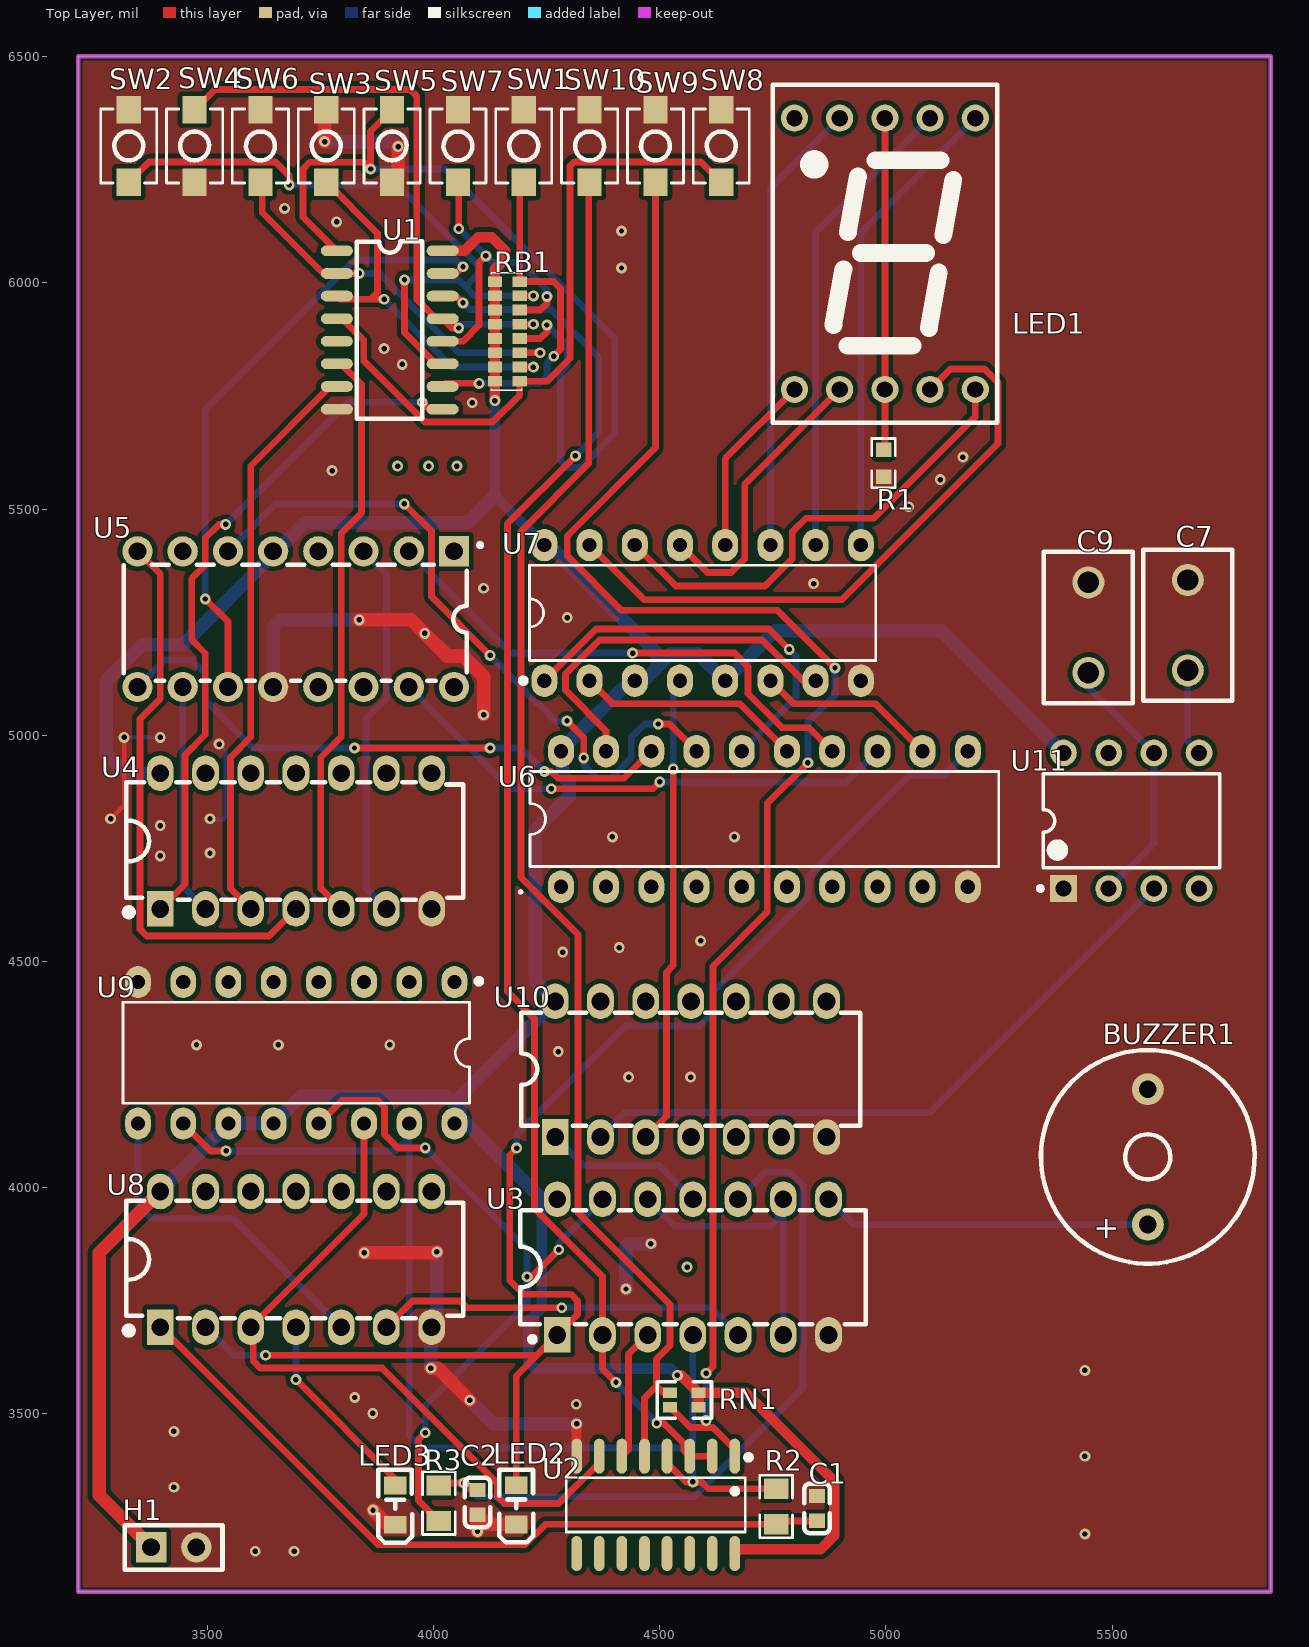
[diagram p0: Top Layer view]
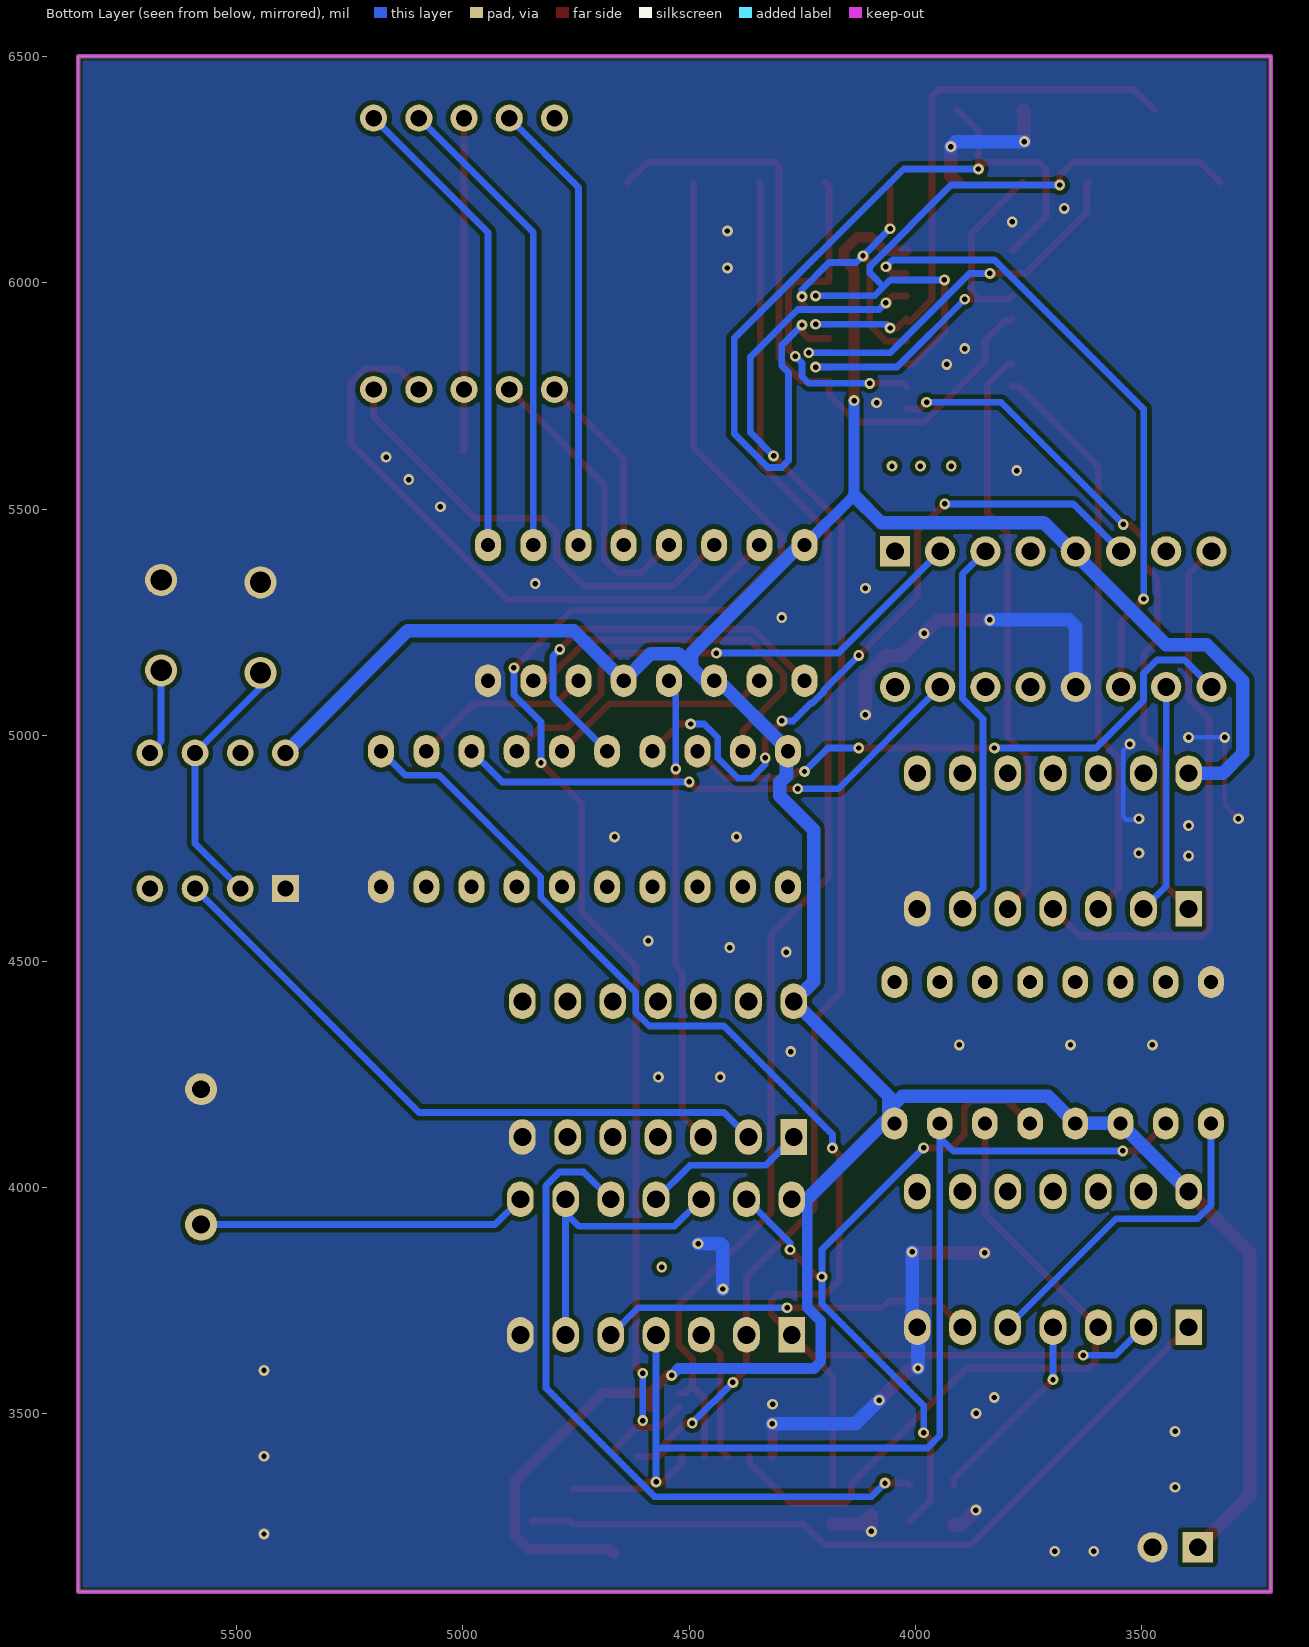
[diagram p1: Bottom Layer view, seen from below]
# Altium PCB MISC51700.pcbdoc
Units mil, origin at the board's own origin, x right, y up, seen from the top; angles counter-clockwise.
Board outline 2638.01 x 3396.77 mil, 2 copper layers (Top Layer, Bottom Layer), stack 62.206 mil thick; 35 components, 54 nets, 236 pads, 115 vias.

## Layer stack, top to bottom
Top Solder Mask Layer: solder mask 0.394, Dk 3.3
Top Layer: signal copper 1.379
Dielectric1: surface 59.449, FR4, Dk 4.5
Bottom Layer: signal copper 1.378
Bottom Solder Mask Layer: solder mask 0.394, Dk 3.3

## Board outline
3213.17,6501.82 3213.17,3105.05 5851.18,3105.05 5851.18,6501.82

## Design rules (kind name [scope] priority, off if disabled: settings)
BoardOutlineClearance copperThickness2oz_1 [All] p2 off: genericclearance=8 ignorepadtopadclearanceinfootprint=FALSE except(0: Arc-SplitContinuation Track-SplitContinuation SMDPad-SplitContinuation THPad-SplitContinuation Via-SplitContinuation Fill-SplitContinuation Region-SplitContinuation Poly-SplitContinuation Text-SplitContinuation Hole-SplitContinuation; 6: Arc-CutoutEdge Track-CutoutEdge SMDPad-CutoutEdge THPad-CutoutEdge Via-CutoutEdge Text-CutoutEdge; 6.9: Hole-OutlineEdge Hole-CutoutEdge; 10: Poly-OutlineEdge Poly-CutoutEdge; 11.8: Arc-OutlineEdge Track-OutlineEdge SMDPad-OutlineEdge THPad-OutlineEdge Via-OutlineEdge Fill-OutlineEdge Region-OutlineEdge Text-OutlineEdge Fill-CutoutEdge Region-CutoutEdge)
BoardOutlineClearance Plane_innerPlane_1 [All] p4 off: genericclearance=4 ignorepadtopadclearanceinfootprint=FALSE except(0: Arc-SplitContinuation Track-SplitContinuation SMDPad-SplitContinuation THPad-SplitContinuation Via-SplitContinuation Fill-SplitContinuation Region-SplitContinuation Poly-SplitContinuation Text-SplitContinuation Hole-SplitContinuation; 6: Arc-CutoutEdge Track-CutoutEdge SMDPad-CutoutEdge THPad-CutoutEdge Via-CutoutEdge Text-CutoutEdge; 6.9: Hole-OutlineEdge Hole-CutoutEdge; 10: Poly-OutlineEdge Poly-CutoutEdge; 11.8: Arc-OutlineEdge Track-OutlineEdge SMDPad-OutlineEdge THPad-OutlineEdge Via-OutlineEdge Fill-OutlineEdge Region-OutlineEdge Text-OutlineEdge Fill-CutoutEdge Region-CutoutEdge)
BoardOutlineClearance Copper_copperRegion_1 [All] p6 off: genericclearance=4 ignorepadtopadclearanceinfootprint=FALSE except(0: Arc-SplitContinuation Track-SplitContinuation SMDPad-SplitContinuation THPad-SplitContinuation Via-SplitContinuation Fill-SplitContinuation Region-SplitContinuation Poly-SplitContinuation Text-SplitContinuation Hole-SplitContinuation; 6: Arc-CutoutEdge Track-CutoutEdge SMDPad-CutoutEdge THPad-CutoutEdge Via-CutoutEdge Text-CutoutEdge; 6.9: Hole-OutlineEdge Hole-CutoutEdge; 10: Poly-OutlineEdge Poly-CutoutEdge; 11.8: Arc-OutlineEdge Track-OutlineEdge SMDPad-OutlineEdge THPad-OutlineEdge Via-OutlineEdge Fill-OutlineEdge Region-OutlineEdge Text-OutlineEdge Fill-CutoutEdge Region-CutoutEdge)
BoardOutlineClearance copperThickness1oz_1 [All] p8: genericclearance=4 ignorepadtopadclearanceinfootprint=FALSE except(0: Arc-SplitContinuation Track-SplitContinuation SMDPad-SplitContinuation THPad-SplitContinuation Via-SplitContinuation Fill-SplitContinuation Region-SplitContinuation Poly-SplitContinuation Text-SplitContinuation Hole-SplitContinuation; 6: Arc-CutoutEdge Track-CutoutEdge SMDPad-CutoutEdge THPad-CutoutEdge Via-CutoutEdge Text-CutoutEdge; 6.9: Hole-OutlineEdge Hole-CutoutEdge; 10: Poly-OutlineEdge Poly-CutoutEdge; 11.8: Arc-OutlineEdge Track-OutlineEdge SMDPad-OutlineEdge THPad-OutlineEdge Via-OutlineEdge Fill-OutlineEdge Region-OutlineEdge Text-OutlineEdge Fill-CutoutEdge Region-CutoutEdge)
Clearance copperThickness2oz [All] p1 off: gap=8 ignorepadtopadclearanceinfootprint=FALSE except(6: SMDPad-Track SMDPad-SMDPad THPad-Track SMDPad-THPad THPad-THPad Track-Via SMDPad-Via THPad-Via Via-Via Fill-SMDPad Region-SMDPad Fill-THPad Region-THPad Fill-Via Region-Via Fill-Fill Fill-Region Region-Region Arc-Track Arc-SMDPad Arc-THPad Arc-Via Fill-Arc Region-Arc Arc-Arc Text-Track SMDPad-Text Text-THPad Text-Via Fill-Text Region-Text Arc-Text Text-Text; 6.9: Hole-Track Hole-SMDPad Hole-THPad Hole-Via Fill-Hole Region-Hole Hole-Arc Hole-Text; 10: Poly-Track Poly-SMDPad Poly-THPad Poly-Via Poly-Fill Poly-Region Poly-Poly Poly-Arc Poly-Text Poly-Hole; 11.8: Fill-Track Region-Track)
Clearance Plane_innerPlane [All] p3 off: gap=4 ignorepadtopadclearanceinfootprint=FALSE except(6: SMDPad-Track SMDPad-SMDPad THPad-Track SMDPad-THPad THPad-THPad Track-Via SMDPad-Via THPad-Via Via-Via Fill-SMDPad Region-SMDPad Fill-THPad Region-THPad Fill-Via Region-Via Fill-Fill Fill-Region Region-Region Arc-Track Arc-SMDPad Arc-THPad Arc-Via Fill-Arc Region-Arc Arc-Arc Text-Track SMDPad-Text Text-THPad Text-Via Fill-Text Region-Text Arc-Text Text-Text; 6.9: Hole-Track Hole-SMDPad Hole-THPad Hole-Via Fill-Hole Region-Hole Hole-Arc Hole-Text; 10: Poly-Track Poly-SMDPad Poly-THPad Poly-Via Poly-Fill Poly-Region Poly-Poly Poly-Arc Poly-Text Poly-Hole; 11.8: Fill-Track Region-Track)
Clearance Copper_copperRegion [All] p5 off: gap=4 ignorepadtopadclearanceinfootprint=FALSE except(6: SMDPad-Track SMDPad-SMDPad THPad-Track SMDPad-THPad THPad-THPad Track-Via SMDPad-Via THPad-Via Via-Via Fill-SMDPad Region-SMDPad Fill-THPad Region-THPad Fill-Via Region-Via Fill-Fill Fill-Region Region-Region Arc-Track Arc-SMDPad Arc-THPad Arc-Via Fill-Arc Region-Arc Arc-Arc Text-Track SMDPad-Text Text-THPad Text-Via Fill-Text Region-Text Arc-Text Text-Text; 6.9: Hole-Track Hole-SMDPad Hole-THPad Hole-Via Fill-Hole Region-Hole Hole-Arc Hole-Text; 10: Poly-Track Poly-SMDPad Poly-THPad Poly-Via Poly-Fill Poly-Region Poly-Poly Poly-Arc Poly-Text Poly-Hole; 11.8: Fill-Track Region-Track)
Clearance copperThickness1oz [All] p7: gap=4 ignorepadtopadclearanceinfootprint=FALSE except(6: SMDPad-Track SMDPad-SMDPad THPad-Track SMDPad-THPad THPad-THPad Track-Via SMDPad-Via THPad-Via Via-Via Fill-SMDPad Region-SMDPad Fill-THPad Region-THPad Fill-Via Region-Via Fill-Fill Fill-Region Region-Region Arc-Track Arc-SMDPad Arc-THPad Arc-Via Fill-Arc Region-Arc Arc-Arc Text-Track SMDPad-Text Text-THPad Text-Via Fill-Text Region-Text Arc-Text Text-Text; 6.9: Hole-Track Hole-SMDPad Hole-THPad Hole-Via Fill-Hole Region-Hole Hole-Arc Hole-Text; 10: Poly-Track Poly-SMDPad Poly-THPad Poly-Via Poly-Fill Poly-Region Poly-Poly Poly-Arc Poly-Text Poly-Hole; 11.8: Fill-Track Region-Track)
DiffPairsRouting differentialPair [All] p1: maxlimit=6 minlimit=6 mostfreqgap=6 toplayer_minwidth=5 toplayer_prefwidth=10 toplayer_maxwidth=100 toplayer_mingap=6 toplayer_prefgap=6 toplayer_maxgap=6 bottomlayer_minwidth=5 bottomlayer_prefwidth=10 bottomlayer_maxwidth=100 bottomlayer_mingap=6 bottomlayer_prefgap=6 bottomlayer_maxgap=6 maxuncoupledlength=10
HoleToHoleClearance otherClearance [All] p1: gap=11.8 allowstackedmicrovias=TRUE
Length netLength [All] p1: minlimit=0 maxlimit=0
PasteMaskExpansion pasteMaskExpansion [All] p1: expansion=0
PlaneConnect innerPlane [All] p1: planeconnectstyle=Relief reliefexpansion=20 reliefentries=4 reliefconductorwidth=10 reliefairgap=10
PolygonConnect copperRegion [All] p1: connectstyle=Direct reliefconductorwidth=10 reliefentries=4 polygonreliefangle="90 Angle" airgapwidth=10 via.connectstyle=Relief via.reliefconductorwidth=10 via.reliefentries=4 via.polygonreliefangle="90 Angle" via.airgapwidth=10
RoutingVias viaSize [All] p1: holewidth=12 width=24 viastyle="Through Hole" minholewidth=11.8 minwidth=19.7 maxholewidth=248 maxwidth=393.7
SolderMaskExpansion solderMaskExpansion [IsVia] p1: expansion=-1000 istentingtop=TRUE
SolderMaskExpansion solderMaskExpansion [All] p2: expansion=2 istentingtop=FALSE
Width copperThickness2oz_2 [All] p1 off: maxlimit=100 minlimit=8 preferedwidth=10
Width POWER [(InNet('GND') OR InNet('+5V'))] p2: maxlimit=100 minlimit=5 preferedwidth=30
Width copperThickness1oz_2 [All] p3: maxlimit=100 minlimit=5 preferedwidth=10

## Components (designator, comment, footprint, x,y, rotation, side; value= is the part's Value field where it differs from the comment)
BUZZER1 "2.4kHz" BUZ-TH_BD12.0-P7.60-D0.6-FD 5579.03,4067.26 r90 top
C1 "1uF" C0603 4847.45,3289.76 r90 top
C2 "10uF" C0603 4096.6,3303.08 r90 top
C7 "C104" CAP-TH_L8.5-W5.0-P5.00-D1.2 5667.54,5243.17 r270 top
C9 "C103" CAP-TH_L8.5-W5.0-P5.00-D1.2 5447.64,5237.74 r270 top
H1 "" HDR-TH_2P-P2.54-V-F 3424.71,3203.82 r0 top
LED1 "" LED-SEG-TH_10P-L12.6-W19.0-P2.54-S15.24-BL 4997.53,6064.58 r180 top
LED2 "" LED_0805 4182.51,3299.61 r90 top
LED3 "" LED_0805 3914.72,3298.85 r90 top
R1 "50Ω" R0603 4994.76,5601.45 r90 top
R2 "100K" R0805 4756.93,3293.92 r90 top
R3 "72K" R0805 4011.03,3301.35 r90 top
RB1 "10kΩ" RES-ARRAY-SMD_0603-16P-L6.4-W1.6-TL 4162.57,5892.81 r270 top
RN1 "10kΩ" RES-ARRAY-SMD_0603-4P-L1.6-W1.6-BL 4554.02,3529.58 r90 top
SW1 "" Key_SMD_3x4x2 4198.93,6302.98 r270 top
SW2 "" Key_SMD_3x4x2 3325.3,6302.98 r270 top
SW3 "" Key_SMD_3x4x2 4053.33,6302.98 r270 top
SW4 "" Key_SMD_3x4x2 3470.91,6302.98 r90 top
SW5 "" Key_SMD_3x4x2 3907.72,6302.98 r90 top
SW6 "" Key_SMD_3x4x2 3616.51,6302.98 r270 top
SW7 "" Key_SMD_3x4x2 3762.12,6302.98 r270 top
SW8 "" Key_SMD_3x4x2 4635.74,6302.98 r270 top
SW9 "" Key_SMD_3x4x2 4490.14,6302.98 r270 top
SW10 "" Key_SMD_3x4x2 4344.53,6302.98 r270 top
U1 "SN74LS148DR(LX)" SOIC-16_L9.9-W3.9-P1.27-LS6.0-BL-1 3902.46,5896.05 r270 top
U2 "SN74LS279D" SOIC-16_L9.9-W3.9-P1.27-LS6.0-BL 4490.8,3297.61 r180 top
U3 "SN74LS08N" PDIP-14_L19.3-W6.4-P2.54-LS7.9-BL-1 4572.92,3823.56 r0 top
U4 "SN74LS04N(LX)" DIP-14_L19.1-W6.4-P2.54-LS7.6-BL 3695.04,4765.77 r0 top
U5 "XD74LS83" PDIP-16_L19.1-W6.4-P2.54-LS7.62-BL 3694.54,5256.46 r180 top
U6 "SN74LS373N(LX)" PDIP-20_L26.2-W7.6-P2.54-LS7.9-BL 4731,4814.57 r0 top
U7 "XD74LS48" DIP-16_L19.3-W6.4-P2.54-LS7.6-BL 4594.39,5270.34 r0 top
U8 "SN74LS04N(LX)" DIP-14_L19.1-W6.4-P2.54-LS7.6-BL 3695.04,3840.57 r0 top
U9 "SN74LS279AN(LX)" PDIP-16_L19.3-W6.4-P2.54-LS7.94-BL 3695.64,4297.49 r180 top
U10 "SN74LS00N(XBLW)" PDIP-14_L19.3-W6.4-P2.54-LS7.6-BL 4568.51,4261.19 r0 top
U11 "100kHz" DIP-8_L9.8-W6.6-P2.54-LS7.6-BL 5542.48,4810.61 r0 top

## Footprints (in the part's own frame and the unit in brackets; to place one, negate y for a bottom-side part, rotate by r counter-clockwise, add the part's x,y. Pads: shape width x height; smd on the part's side, far side on the other; paste and mask are expansions set on the pad)
BUZ-TH_BD12.0-P7.60-D0.6-FD [mm]
  round 1.8 hole 1: 1(-3.8,0) 2(3.8,0)
  silkscreen extent -6,-6 6,6
C0603 [mm]
  rect 0.8x0.9 smd: 1(-0.7,0) 2(0.7,0)
  silkscreen extent -1.39,-0.71 1.39,0.71
CAP-TH_L8.5-W5.0-P5.00-D1.2 [mm]
  round 1.8 hole 1.2: 1(-2.54,0) 2(2.54,0)
  silkscreen extent -4.25,-2.5 4.25,2.5
DIP-8_L9.8-W6.6-P2.54-LS7.6-BL [mm]
  rect 1.5x1.5 hole 0.9: 1(-3.81,-3.81)
  round 1.5 hole 0.9: 2(-1.27,-3.81) 3(1.27,-3.81) 4(3.81,-3.81) 5(3.81,3.81) 6(1.27,3.81) 7(-1.27,3.81) 8(-3.81,3.81)
  silkscreen extent -5.23,-3.93 4.96,2.65
DIP-14_L19.1-W6.4-P2.54-LS7.6-BL [mm]
  rect 1.5x2 hole 1: 1(-7.62,-3.81)
  oval 1.5x2 hole 1: 2(-5.08,-3.81) 3(-2.54,-3.81) 4(0,-3.81) 5(2.54,-3.81) 6(5.08,-3.81) 7(7.62,-3.81) 8(7.62,3.81) 9(5.08,3.81) 10(2.54,3.81) 11(0,3.81) 12(-2.54,3.81) 13(-5.08,3.81) 14(-7.62,3.81)
  silkscreen extent -9.59,-4.2 9.4,3.3
DIP-16_L19.3-W6.4-P2.54-LS7.6-BL [mm]
  oval 1.46x1.825 hole 0.8: 1(-8.89,-3.81) 2(-6.35,-3.81) 3(-3.81,-3.81) 4(-1.27,-3.81) 5(1.27,-3.81) 6(3.81,-3.81) 7(6.35,-3.81) 8(8.89,-3.81) 9(8.89,3.81) 10(6.35,3.81) 11(3.81,3.81) 12(1.27,3.81) 13(-1.27,3.81) 14(-3.81,3.81) 15(-6.35,3.81) 16(-8.89,3.81)
  silkscreen extent -10.22,-3.96 9.73,2.67
HDR-TH_2P-P2.54-V-F [mm]
  rect 1.7x1.7 hole 1: 1(-1.27,0)
  round 1.7 hole 1: 2(1.27,0)
  silkscreen extent -2.74,-1.25 2.74,1.25
Key_SMD_3x4x2 [mm]
  rect 1.53x1.36 smd paste+0 mask+0.051: 1(-2.035,0) 2(2.035,0)
  silkscreen extent -2.08,-1.58 2.08,1.58
LED-SEG-TH_10P-L12.6-W19.0-P2.54-S15.24-BL [mil]
  round 60 hole 36: 1(-200,-300) 2(-100,-300) 3(0,-300) 4(100,-300) 5(200,-300) 6(200,300) 7(100,300) 8(0,300) 9(-100,300) 10(-200,300)
  silkscreen extent -248,-374 248,374
LED_0805 [mm]
  rect 1x1.25 smd paste+0 mask+0.051: 1(-1.15,0.005) 2(1.05,0.005)
  silkscreen extent -2.15,-0.94 1.93,0.97
PDIP-14_L19.3-W6.4-P2.54-LS7.6-BL [mm]
  rect 1.5x2 hole 1: 1(-7.62,-3.81)
  oval 1.5x2 hole 1: 2(-5.08,-3.81) 3(-2.54,-3.81) 4(0,-3.81) 5(2.54,-3.81) 6(5.08,-3.81) 7(7.62,-3.81) 8(7.62,3.81) 9(5.08,3.81) 10(2.54,3.81) 11(0,3.81) 12(-2.54,3.81) 13(-5.08,3.81) 14(-7.62,3.81)
  silkscreen extent -9.53,-3.17 9.53,3.17
PDIP-14_L19.3-W6.4-P2.54-LS7.9-BL-1 [mm]
  rect 1.5x2 hole 1: 1(-7.62,-3.81)
  oval 1.5x2 hole 1: 2(-5.08,-3.81) 3(-2.54,-3.81) 4(0,-3.81) 5(2.54,-3.81) 6(5.08,-3.81) 7(7.62,-3.81)
  oval 1.5x2 hole 1 copper offset 0,0: 8(7.62,3.81) 9(5.08,3.81) 10(2.54,3.81) 11(0,3.81) 12(-2.54,3.81) 13(-5.08,3.81) 14(-7.62,3.81)
  silkscreen extent -9.7,-4.21 9.7,3.2
PDIP-16_L19.1-W6.4-P2.54-LS7.62-BL [mm]
  rect 1.7x1.7 hole 1: 1(-8.89,-3.81)
  round 1.7 hole 1: 2(-6.35,-3.81) 3(-3.81,-3.81) 4(-1.27,-3.81) 5(1.27,-3.81) 6(3.81,-3.81) 7(6.35,-3.81) 8(8.89,-3.81) 9(8.89,3.81) 10(6.35,3.81) 11(3.81,3.81) 12(1.27,3.81) 13(-1.27,3.81) 14(-3.81,3.81) 15(-6.35,3.81) 16(-8.89,3.81)
  silkscreen extent -10.46,-4.26 9.65,3.46
PDIP-16_L19.3-W6.4-P2.54-LS7.94-BL [mm]
  oval 1.44x1.8 hole 0.8: 1(-8.89,-3.97) 2(-6.35,-3.97) 3(-3.81,-3.97) 4(-1.27,-3.97) 5(1.27,-3.97) 6(3.81,-3.97) 7(6.35,-3.97) 8(8.89,-3.97) 9(8.89,3.97) 10(6.35,3.97) 11(3.81,3.97) 12(1.27,3.97) 13(-1.27,3.97) 14(-3.81,3.97) 15(-6.35,3.97) 16(-8.89,3.97)
  silkscreen extent -10.41,-4.17 9.73,2.84
PDIP-20_L26.2-W7.6-P2.54-LS7.9-BL [mm]
  oval 1.46x1.825 hole 0.8: 1(-11.43,-3.81) 2(-8.89,-3.81) 3(-6.35,-3.81) 4(-3.81,-3.81) 5(-1.27,-3.81) 6(1.27,-3.81) 7(3.81,-3.81) 8(6.35,-3.81) 9(8.89,-3.81) 10(11.43,-3.81) 11(11.43,3.81) 12(8.89,3.81) 13(6.35,3.81) 14(3.81,3.81) 15(1.27,3.81) 16(-1.27,3.81) 17(-3.81,3.81) 18(-6.35,3.81) 19(-8.89,3.81) 20(-11.43,3.81)
  silkscreen extent -13.77,-4.17 13.17,2.67
R0603 [mil]
  rect 31.75x34.02 smd paste-3937.01 mask+2: 1(-29.66,0) 2(29.66,0)
  silkscreen extent -55,-26 55,26
R0805 [mm]
  rect 1.133x1.377 smd paste-100 mask+0.051: 1(-1,0) 2(1,0)
  silkscreen extent -1.76,-0.92 1.76,0.92
RES-ARRAY-SMD_0603-4P-L1.6-W1.6-BL [mm]
  rect 0.6x0.8 smd: 1(-0.4,-0.8) 2(0.4,-0.8) 3(0.4,0.8) 4(-0.4,0.8)
  silkscreen extent -1.02,-1.52 1.02,1.52
RES-ARRAY-SMD_0603-16P-L6.4-W1.6-TL [mm]
  rect 0.6x0.8 smd paste+0 mask+0.05: 1(-2.8,0.7) 2(-2,0.7) 3(-1.2,0.7) 4(-0.4,0.7) 5(0.4,0.7) 6(1.2,0.7) 7(2,0.7) 8(2.8,0.7) 9(2.8,-0.7) 10(2,-0.7) 11(1.2,-0.7) 12(0.4,-0.7) 13(-0.4,-0.7) 14(-1.2,-0.7) 15(-2,-0.7) 16(-2.8,-0.7)
  silkscreen extent -3.3,-0.9 3.3,0.8
SOIC-16_L9.9-W3.9-P1.27-LS6.0-BL [mil]
  oval 23.7x77.6 smd: 1(-175,-107.7) 2(-125,-107.7) 3(-75,-107.7) 4(-25,-107.7) 5(25,-107.7) 6(75,-107.7) 7(125,-107.7) 8(175,-107.7) 9(175,107.7) 10(125,107.7) 11(75,107.7) 12(25,107.7) 13(-25,107.7) 14(-75,107.7) 15(-125,107.7) 16(-175,107.7)
  silkscreen extent -211,-111 198,60
SOIC-16_L9.9-W3.9-P1.27-LS6.0-BL-1 [mm]
  oval 0.6x1.8 smd: 1(-4.445,-2.972) 2(-3.175,-2.972) 3(-1.905,-2.972) 4(-0.635,-2.972) 5(0.635,-2.972) 6(1.905,-2.972) 7(3.175,-2.972) 8(4.445,-2.972) 9(4.445,2.972) 10(3.175,2.972) 11(1.905,2.972) 12(0.635,2.972) 13(-0.635,2.972) 14(-1.905,2.972) 15(-3.175,2.972) 16(-4.445,2.972)
  silkscreen extent -4.98,-1.85 4.98,1.83

## Via types
v1: diameter 24, hole 12, Top Layer to Bottom Layer, 115 vias

## Nets (pads, with @x,y where several pads share a name; then routed paths per layer and width w, separated by ;. In a path a pad name is that pad's centre, name@x,y a point inside that pad or via, vN(x,y) a via of type N, cw(c..) or ccw(c..) an arc to the next point about the centre after c; other vN are vias at no path point)
$1N8479: RB1.1 SW1.2 U1.10 | length 766.9
  Top Layer w15: U1.10 4026.46,5778.05 v1(4100.12,5778.05) ; SW1.2 4190.12,6214.06 RB1.1 4265.12,6003.05 4280.12,5988.05 4280.12,5853.05 v1(4265.12,5838.05)
  Bottom Layer w15: v1(4100.12,5778.05) 4235.12,5778.05 4250.12,5793.05 4250.12,5823.05 v1(4265.12,5838.05)
$1N8484: RB1.2 SW2.2 U1.11 | length 1518
  Top Layer w15: SW2.2 3370.3,6267.86 3650.12,6267.86 3680.12,6237.86 v1(3680.12,6216.71) ; v1(3935.12,6006.71) 3935.12,5890.39 4004.46,5821.05 U1.11 ; RB1.2 v1(4220.12,5971.55)
  Bottom Layer w15: v1(3680.12,6216.71) 3920.12,6216.71 4100.12,6036.71 4100.12,6021.71 4070.12,5991.71 ; v1(3935.12,6006.71) 4055.12,6006.71 4070.12,5991.71 ; v1(4220.12,5971.55) 4090.29,5971.55 4070.12,5991.71
$1N8491: RB1.3 SW3.2 U1.12 | length 705.7
  Top Layer w15: U1.12 4064.46,5871.05 4100.12,5906.71 4100.12,6045.05 v1(4115.12,6060.05) ; SW3.2 4055.12,6221.06 v1(4055.12,6120.05) ; RB1.3 4235.12,5940.05 4250.12,5955.05 v1(4250.12,5970.05)
  Bottom Layer w15: v1(4055.12,6120.05) v1(4115.12,6060.05) 4130.12,6045.05 4190.12,6045.05 4250.12,5985.05 v1(4250.12,5970.05)
$1N8497: RB1.4 SW4.2 U1.13 | length 1291.4
  Top Layer w15: SW4.2 3515.91,6428.1 3947.41,6428.1 3962.41,6413.1 3962.41,5963.1 4010.12,5915.39 U1.13@4025.12,5915.39 ; U1.13 U1.13@4025.12,5915.39 ; v1(4055.12,5900.39) 4040.12,5900.39 U1.13@4025.12,5915.39 ; RB1.4 v1(4220.12,5908.56)
  Bottom Layer w15: v1(4055.12,5900.39) 4063.29,5908.56 v1(4220.12,5908.56)
$1N8503: RB1.5 SW5.2 U1.1 | length 1993.6
  Top Layer w15: U1.1 3710.46,6146.05 3710.46,6252.06 3725.46,6267.06 3845.12,6267.06 v1(3860.12,6252.06) 3860.12,6335.51 SW5.2 ; RB1.5 4235.12,5877.06 4250.12,5892.06 v1(4250.12,5907.06)
  Bottom Layer w15: v1(3860.12,6252.06) 4025.12,6252.06 4400.12,5877.06 4400.12,5667.06 4325.12,5592.06 4295.12,5592.06 4280.12,5607.06 4280.12,5802.06 4295.12,5817.06 4295.12,5862.06 v1(4250.12,5907.06)
$1N8509: RB1.6 SW6.2 U1.2 | length 856.7
  Top Layer w15: SW6.2 3620.46,6218.91 3620.46,6156.05 3755.46,6021.05 U1.2 v1(3834.64,6021.05) ; RB1.6 v1(4235.12,5845.57)
  Bottom Layer w15: v1(3834.64,6021.05) 3879.64,6021.05 4055.12,5845.57 v1(4235.12,5845.57)
$1N8516: RB1.7 SW7.2 U1.3 | length 841.5
  Top Layer w15: SW7.2 3875.12,6109.85 3875.12,5979.07 3860.12,5964.07 ; U1.3 3792.45,5964.07 3860.12,5964.07 ; v1(3890.12,5964.07) 3860.12,5964.07 ; RB1.7 v1(4220.12,5814.07)
  Bottom Layer w15: v1(3890.12,5964.07) 4040.12,5814.07 v1(4220.12,5814.07)
$1N8523: RB1.8 SW8.2 U1.4 | length 1494.9
  Top Layer w15: U1.4 3788.95,5917.57 3800.12,5917.57 3845.12,5872.57 3845.12,5827.57 3980.12,5692.57 4130.12,5692.57 4190.12,5752.57 RB1.8 4250.12,5782.57 4301.12,5833.57 4301.12,6258.86 4310.12,6267.86 4590.74,6267.86 SW8.2
$1N9036: RN1.4 SW9.2 U2.1 | length 3597.2
  Top Layer w15: SW9.2 4490.14,5635.97 4295.14,5440.97 4295.14,5395.97 4415.14,5275.97 4760.14,5275.97 v1(4887.28,5148.83) ; RN1.4 4567.52,3468.83 4602.28,3468.83 ; v1(4602.28,3483.83) 4602.28,3468.83 ; v1(4602.28,3588.83) 4617.28,3603.83 4617.28,4488.83 4737.28,4608.83 4737.28,4848.83 v1(4827.28,4938.83) ; U2.1 4662.28,3408.83 4662.28,3423.83 4617.28,3468.83 4602.28,3468.83
  Bottom Layer w15: v1(4602.28,3483.83) v1(4602.28,3588.83) ; v1(4827.28,4938.83) 4827.28,5028.83 4887.28,5088.83 v1(4887.28,5148.83)
$1N9040: RN1.3 SW10.2 U2.5 | length 3076.9
  Top Layer w15: SW10.2 4342.52,6220.85 4342.52,5600.33 4192.52,5450.33 4192.52,4685.33 4318.52,4559.33 4318.52,3944.33 4522.52,3740.33 4522.52,3650.33 4492.52,3620.33 4492.52,3560.33 ; U2.5 4465.8,3533.61 4492.52,3560.33 ; RN1.3 4507.52,3545.33 4492.52,3560.33
$1N9149: U1.14 U2.2 U2.3 U3.2 | length 3140.8
  Top Layer w15: U1.14 4049.46,5971.05 v1(4064.46,5956.05) ; v1(4312.92,5617.6) 4162.92,5467.6 4162.92,4432.6 4222.92,4372.6 4222.92,3952.6 4372.92,3802.6 U3.2 4372.92,3598.56 v1(4402.92,3568.56) ; v1(4492.92,3478.56) 4507.92,3478.56 4552.92,3433.56 4552.92,3418.19 U2.3 U2.2
  Bottom Layer w15: v1(4064.46,5956.05) 4079.46,5941.05 4259.46,5941.05 4364.46,5836.05 4364.46,5669.15 v1(4312.92,5617.6) ; v1(4402.92,3568.56) v1(4492.92,3478.56)
$1N9245: U2.6 U3.3 | length 291.9
  Top Layer w15: U2.6 4430.8,3420.31 4430.8,3631.44 U3.3
$1N9427: U1.9 U4.1 | length 1541.8
  Top Layer w15: U4.1 3449.46,4670.2 3449.46,4956.05 3494.46,5001.05 3494.46,5181.05 3464.46,5211.05 3464.46,5346.05 3494.46,5376.05 3494.46,5436.05 3524.46,5466.05 v1(3539.46,5466.05) ; v1(3974.46,5736.05) 3989.46,5721.05 U1.9
  Bottom Layer w15: v1(3539.46,5466.05) 3809.46,5736.05 v1(3974.46,5736.05)
$1N9583: U4.2 U5.10 | length 511.6
  Bottom Layer w15: U5.10 3444.54,4666.28 U4.2
$1N9591: U1.7 U4.3 | length 1280.2
  Top Layer w15: U4.3 3550.04,4660.77 3550.04,4950.63 3595.04,4995.63 3595.04,5595.63 3770.46,5771.05 U1.7
$1N9600: U4.4 U5.8 | length 1251.3
  Top Layer w15: U5.8 3395.04,5355.95 3395.04,5080.77 3350.04,5035.77 3350.04,4570.77 3365.04,4555.77 3635.04,4555.77 U4.4
$1N9611: U1.6 U4.5 | length 1289.4
  Top Layer w15: U1.6 3795.04,5821.05 3840.04,5776.05 3840.04,5491.05 3795.04,5446.05 3795.04,4996.05 3750.04,4951.05 3750.04,4660.77 U4.5
$1N9618: U4.6 U5.3 | length 848.9
  Bottom Layer w15: U5.3 3895.04,5355.95 3895.04,5080.77 3850.04,5035.77 3850.04,4660.77 U4.6
$1N9631: U1.15 U5.11 | length 1399.5
  Top Layer w15: v1(3494.46,5301.05) 3544.54,5250.98 U5.11 ; U1.15 4049.46,6021.05 v1(4064.46,6036.05)
  Bottom Layer w15: v1(3494.46,5301.05) 3494.46,5721.05 3824.46,6051.05 4049.46,6051.05 v1(4064.46,6036.05)
$1N9827: U5.15 U6.13 | length 1164.1
  Top Layer w15: v1(4259.54,4881.46) 4484.54,4881.46 v1(4499.54,4896.46)
  Bottom Layer w15: U5.15 4169.54,4881.46 v1(4259.54,4881.46) ; v1(4499.54,4896.46) 4912.89,4896.46 U6.13
$1N9833: U5.2 U6.14 | length 1154.6
  Top Layer w15: v1(4439.54,5181.46) 4664.54,5181.46 4694.54,5151.46 4694.54,5091.46 4769.54,5016.46 4829.11,5016.46 U6.14
  Bottom Layer w15: U5.2 4169.54,5181.46 v1(4439.54,5181.46)
$1N9838: U5.6 U6.17 | length 1554.2
  Top Layer w15: v1(3934.54,5511.46) 3994.54,5451.46 3994.54,5306.46 v1(4124.54,5176.46) ; v1(4294.54,5031.46) 4331.43,4994.57 v1(4331.43,4949.57) ; v1(4496.43,5024.57) 4521,5024.57 U6.17
  Bottom Layer w15: U5.6 3649.54,5511.46 v1(3934.54,5511.46) ; v1(4124.54,5176.46) 4202.15,5098.84 4202.15,5095.66 4226.9,5070.92 4230.08,5070.92 4269.54,5031.46 v1(4294.54,5031.46) ; v1(4331.43,4949.57) 4331.43,4934.57 4361.43,4904.57 4391.43,4904.57 4436.43,4949.57 4436.43,4994.57 4466.43,5024.57 v1(4496.43,5024.57)
$1N9844: U5.9 U6.18 | length 1329.8
  Top Layer w15: v1(3824.54,4971.46) v1(4124.54,4971.46) ; v1(4244.54,4919.57) 4259.54,4919.57 4274.54,4904.57 4421,4904.57 U6.18
  Bottom Layer w15: U5.9 3404.54,5166.46 3464.54,5166.46 3494.54,5136.46 3494.54,5076.46 3599.54,4971.46 v1(3824.54,4971.46) ; v1(4124.54,4971.46) 4192.65,4971.46 v1(4244.54,4919.57)
$1N9926: U6.19 U7.7 | length 829.8
  Top Layer w15: U6.19 4381,5009.57 4291,5099.57 4291,5135.34 4366,5210.34 4726,5210.34 4816,5120.34 U7.7
$1N9939: U6.16 U7.1 | length 888.5
  Top Layer w15: U7.1 4358.62,5234.57 4741,5234.57 v1(4786,5189.57)
  Bottom Layer w15: U6.16 4801,5084.57 4801,5174.57 v1(4786,5189.57)
$1N9972: U6.15 U7.2 | length 501.1
  Top Layer w15: U7.2 4395.17,5069.57 4676,5069.57 U6.15
$1N9987: U6.12 U7.6 | length 401.1
  Top Layer w15: U7.6 4795.17,5069.57 4976,5069.57 U6.12
$1N10140: LED1.1 U7.9 | length 1049.1
  Bottom Layer w15: U7.9 4944.39,6111.44 LED1.1
$1N10149: LED1.2 U7.10 | length 1049.1
  Bottom Layer w15: U7.10 4844.39,6111.44 LED1.2
$1N10162: LED1.4 U7.11 | length 1007.7
  Bottom Layer w15: U7.11 4744.39,6211.44 LED1.4
$1N10172: LED1.6 U7.12 | length 407.7
  Top Layer w15: U7.12 4644.39,5611.44 LED1.6
$1N10182: LED1.7 U7.13 | length 642.7
  Top Layer w15: U7.13 4605.16,5359.58 4657.53,5359.58 4687.53,5389.58 4687.53,5554.58 LED1.7
$1N10192: LED1.10 U7.14 | length 1041.2
  Top Layer w15: U7.14 4535.16,5329.58 4732.53,5329.58 4792.53,5389.58 4792.53,5449.58 4822.53,5479.58 4972.53,5479.58 5197.53,5704.58 LED1.10
$1N10216: LED1.9 U7.15 | length 1412.1
  Top Layer w15: U7.15 4465.16,5299.58 4902.53,5299.58 5247.53,5644.58 5247.53,5779.58 5217.53,5809.58 5142.53,5809.58 LED1.9
$1N10246: LED1.3 LED1.8 R1.2 | length 737.7
  Top Layer w15: LED1.3 LED1.8 4997.53,5630 R1.2@4999.75,5627.78
$1N10358: R2.2 U2.4 U3.4 U9.10 U9.15 | length 2471.7
  Top Layer w15: U9.10 3506.35,4080.47 v1(3540.64,4080.47) ; U2.4 4515.8,3390.31 4557.82,3348.29 v1(4572.82,3348.29) 4591.93,3348.29 4606.93,3333.29 R2.2
  Bottom Layer w15: v1(3540.64,4080.47) 3915.64,4080.47 U9.15@3945.64,4110.47 ; U9.15 U9.15@3945.64,4110.47 ; v1(4572.82,3348.29) U3.4@4572.82,3673.47 ; 4572.82,3423.29 3972.82,3423.29 3945.64,3450.47 U9.15@3945.64,4110.47
$1N10490: C1.1 R2.1 U8.1 | length 1673.5
  Top Layer w15: U8.1 3876.06,3209.55 4201.93,3209.55 4246.93,3254.55 R2.1 4764.58,3262.2 C1.1
$1N10518: LED2.2 U3.1 U6.11 U8.2 | length 3122.2
  Top Layer w15: v1(3627.92,3628.57) 4227.92,3628.57 ; LED2.2 4182.31,3582.96 4227.92,3628.57 ; v1(4182.92,4086.49) 4167.92,4071.49 4167.92,3793.57 4197.92,3763.57 4302.92,3763.57 4317.92,3748.57 4317.92,3718.57 U3.1 4227.92,3628.57
  Bottom Layer w15: U8.2 3557.04,3628.57 v1(3627.92,3628.57) ; v1(4182.92,4086.49) 4182.92,4116.49 4422.92,4356.49 4587.92,4356.49 4617.92,4386.49 4617.92,4431.49 4827.92,4641.49 4827.92,4686.49 5052.92,4911.49 5127.92,4911.49 U6.11
$1N10779: U2.7 U8.3 U9.14 | length 1597.4
  Top Layer w15: U9.14 3845.64,3941.17 U8.3 3600.8,3684.81 3600.8,3615.31 3615.8,3600.31 3885.8,3600.31 4140.8,3345.31 4140.8,3315.31 4155.8,3300.31 4275.8,3300.31 4365.8,3390.31 U2.7
$1N10824: LED3.2 U8.4 | length 441.3
  Top Layer w15: v1(3695.04,3574.67) 3914.52,3355.19 LED3.2
  Bottom Layer w15: v1(3695.04,3574.67) U8.4
$1N10957: U8.5 U9.9 | length 742.2
  Bottom Layer w15: U9.9 3345.64,3959.98 3375.04,3930.57 3555.04,3930.57 U8.5
$1N10966: U3.5 U8.6 | length 833
  Top Layer w15: U8.6 3953.03,3748.56 4057.92,3748.56 4072.92,3733.56 v1(4282.92,3733.56)
  Bottom Layer w15: v1(4282.92,3733.56) 4612.92,3733.56 U3.5
$1N10980: U3.6 U3.9 U3.12 | length 637.3
  Bottom Layer w15: U3.12 4532.92,3913.56 4742.92,3913.56 U3.9@4772.92,3943.56 ; U3.6 U3.9@4772.92,3943.56 ; U3.9 U3.9@4772.92,3943.56
$1N11033: R3.1 U3.13 U9.13 | length 1618.1
  Top Layer w15: U9.13 3796.43,4191.98 3876.03,4191.98 3891.03,4176.98 3891.03,4116.98 3921.03,4086.98 v1(3981.03,4086.98) ; v1(3981.03,3456.98) 3966.03,3441.98 3966.03,3306.98 R3.1 ; v1(4206.03,3801.98) 4216.33,3801.98 v1(4276.33,3861.98)
  Bottom Layer w15: v1(3981.03,3456.98) 3981.03,3516.98 4206.03,3741.98 v1(4206.03,3801.98) 4206.03,3861.98 v1(3981.03,4086.98) ; v1(4276.33,3861.98) 4276.33,3876.98 U3.13
$1N11083: C2.2 R3.2 U3.10 | length 1584.5
  Top Layer w15: R3.2 4015.96,3345.64 v1(4066.6,3345.64) 4081.6,3330.64 C2.2
  Bottom Layer w15: v1(4066.6,3345.64) 4096.6,3315.64 4576.6,3315.64 4816.6,3555.64 4816.6,4003.56 4786.6,4033.56 4732.92,4033.56 U3.10
$1N11188: BUZZER1.1 U3.8 | length 729.3
  Bottom Layer w15: U3.8 4928.82,3917.66 BUZZER1.1
$1N11397: U3.11 U10.1 | length 361.4
  Bottom Layer w15: U10.1 4331.13,4048.56 4497.92,4048.56 U3.11
$1N11407: U7.4 U10.3 | length 1040.6
  Top Layer w15: U10.3 4514.39,4157.07 4514.39,4475.34 4529.39,4490.34 v1(4529.39,4925.34)
  Bottom Layer w15: v1(4529.39,4925.34) 4529.39,5105.34 U7.4
$1N11538: C9.2 U11.2 U11.6 | length 578.5
  Bottom Layer w15: C9.2 5447.64,5105.45 U11.6 5592.48,4760.61 U11.2
$1N11539: U11.4
$1N11594: C7.2 U11.5 | length 192.9
  Bottom Layer w15: C7.2 5667.54,4985.55 U11.5
$1N11600: U10.2 U11.3 | length 1451.5
  Bottom Layer w15: U10.2 4422.94,4165.61 5097.48,4165.61 U11.3
+5V: H1.1 RB1.9 RB1.10 RB1.11 RB1.12 RB1.13 RB1.14 RB1.15 RB1.16 RN1.1 RN1.2 U1.16 U2.16 U3.14 U4.14 U5.5 U6.20 U7.3 U7.5 U7.16 U8.14 U9.11 U9.12 U9.16 U10.14 U11.8 | length 8438.5
  Top Layer w23.62: U1.16 4067.95,6071.05 4097.95,6101.05 4127.95,6101.05 4157.95,6071.05 4157.95,6052.57 4135,6029.63 RB1.16 RB1.15 RB1.14 RB1.13 RB1.12 RB1.11 RB1.10 RB1.9 v1(4135,5739.73) ; v1(4538.51,3584.06) 4546.79,3584.06 RN1.2 ; RN1.1 RN1.2 ; U2.16 4675.51,3199.62 4855.51,3199.62 4885.51,3229.62 4885.51,3349.62 4689.8,3545.33 RN1.2
  Top Layer w30: H1.1 3259.77,3318.76 3259.77,3855.29 U8.14
  Bottom Layer w23.62: v1(4135,5739.73) 4135,5529.73 U7.16 ; 4238.51,3974.06 4238.51,3734.06 4208.51,3704.06 4208.51,3614.06 4223.51,3599.06 4523.51,3599.06 v1(4538.51,3584.06)
  Bottom Layer w30: U8.14 U9.11 ; U4.14 3319.23,4915.77 3275.04,4959.96 3275.04,5119.77 3355,5199.73 3445,5199.73 U5.5@3655,5409.73 ; U9.11 U9.12 3705.64,4201.19 4028.51,4201.19 U9.16@4058.51,4171.19 ; U5.5 3647.82,5409.73 U5.5@3655,5409.73 ; U9.16 U9.16@4058.51,4154.06 ; 4135,5529.73 4075,5469.73 3715,5469.73 U5.5@3655,5409.73 ; U7.16 4254.39,5420.34 4494.39,5180.34 4494.39,5150.34 ; U3.14 4272.42,3974.06 4238.51,3974.06 U9.16@4058.51,4154.06 ; U6.20 U6.20@4284.39,4970.34 ; U11.8 5122.48,5230.61 4754.66,5230.61 U7.5 4584.39,5180.34 4524.39,5180.34 4494.39,5150.34 ; U9.16@4058.51,4154.06 U9.16@4058.51,4171.19 ; U9.16@4058.51,4171.19 4058.51,4201.19 U10.14 4224.39,4455.3 4224.39,4790.34 4299.39,4865.34 4299.39,4895.34 4284.39,4910.34 U6.20@4284.39,4970.34 ; U6.20@4284.39,4970.34 4434.39,5120.34 4464.39,5120.34 4494.39,5150.34
GND: BUZZER1.2 C1.2 C2.1 C7.1 C9.1 H1.2 LED2.1 LED3.1 R1.1 SW1.1 SW2.1 SW3.1 SW4.1 SW5.1 SW6.1 SW7.1 SW8.1 SW9.1 SW10.1 U1.8 U2.8 U3.7 U4.7 U5.12 U6.10 U7.8 U8.7 U9.8 U10.7 U11.1 | length 2757.3
  Top Layer w10: v1(3285,4815) 3315,4845 v1(3315,4995)
  Top Layer w22: U2.8 v1(4315.8,3477.05)
  Top Layer w30: v1(3758.3,6312.59) 3758.3,6379.29 SW7.1 ; v1(3835,5255) 3950,5255 v1(3980,5225) 4030,5175 4065,5175 4110,5130 v1(4110,5045) ; v1(3846.19,3854.81) 4004.39,3854.81 v1(4006.61,3857.03) ; v1(3865.51,3286.08) 3898.02,3253.57 LED3.1 ; SW5.1 3920.93,6236.08 v1(3920.93,6301.5) ; v1(3993.56,3599.63) 4008.96,3599.63 v1(4079.52,3529.06) ; v1(4096.6,3238.77) C2.1 4117.79,3254.33 LED2.1
  Bottom Layer w10: v1(3315,4995) v1(3395,4995) ; v1(3505,4815) 3507.07,4812.93 3532.93,4812.93 3540,4820 3540,4965 v1(3525,4980)
  Bottom Layer w30: U5.12 3644.54,5239.54 3660,5255 v1(3835,5255) ; v1(3758.3,6312.59) 3909.85,6312.59 v1(3920.93,6301.5) ; v1(3993.56,3599.63) 3993.56,3689.08 U8.7 4006.61,3702.14 v1(4006.61,3857.03) ; v1(4079.52,3529.06) 4131.53,3477.05 v1(4315.8,3477.05) ; v1(4425,3775) 4425,3870 4430,3875 v1(4480,3875)
  other v1: 3605,3195 3690.97,3195 5440,3233.1 3425,3336.69 5440,3405.05 3425,3460 3865,3500 4315,3520 3825,3535 5440,3595 4430.87,4243.53 4567.78,4243.53 4275,4300 3475,4315 3656.26,4315 3902.35,4315 4285,4520 4410,4530 4590,4545 3395,4732.76 3505,4739.07 4395,4775 4664.61,4775 3395,4800 4295,5260 4110,5325 4840,5335 5050,5505 5120,5565 3775,5585 5170,5615 4085,5735 3930,5820 3890,5855 4415,6033.13 4415,6115 3785,6135 3670,6165
pads on no net: LED1.5 U1.5 U2.9 U2.10 U2.11 U2.12 U2.13 U2.14 U2.15 U4.8 U4.9 U4.10 U4.11 U4.12 U4.13 U5.1 U5.4 U5.7 U5.13 U5.14 U5.16 U6.1 U6.2 U6.3 U6.4 U6.5 U6.6 U6.7 U6.8 U6.9 U8.8 U8.9 U8.10 U8.11 U8.12 U8.13 U9.1 U9.2 U9.3 U9.4 U9.5 U9.6 U9.7 U10.4 U10.5 U10.6 U10.8 U10.9 U10.10 U10.11 U10.12 U10.13 U11.7
copper on no net:
  other v1: 4560.23,3823.56 3920,5595 3988.38,5595 4051.01,5595

## Polygon pours and split planes (outlines as drawn)
GND on Top Layer (solid, remove dead copper, pour order 0): 3125,6615 3125,3015 5960,3015 5960,6615
GND on Bottom Layer (solid, remove dead copper, pour order 2): 3000,6735 3000,3000 6075,3000 6075,6735

## Keep-outs
Board Outline Layer:
  the board outline again, w10